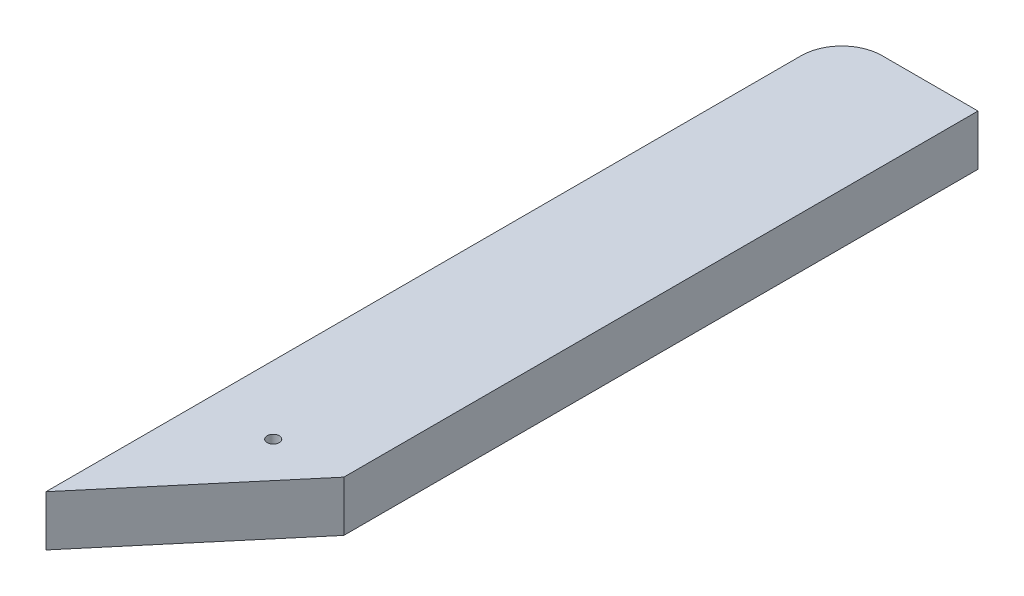
SolidWorks part; units mm, degrees
ref_plane "Front Plane" through (0, 0, 0) normal (0, 0, 1) x (1, 0, 0)
ref_plane "Top Plane" through (0, 0, 0) normal (0, 1, 0) x (1, 0, 0)
ref_plane "Right Plane" through (0, 0, 0) normal (1, 0, 0) x (0, 0, -1)
sketch "Sketch1" plane through (0, 0, 0) normal (0, 1, 0) x (1, 0, 0)
  line L0 (67.5, 0) -> (0, 0)
  line L1 (0, 0) -> (0, -394.0163)
  line L2 (67.5, 0) -> (67.5, -314.0163)
  line L3 (67.5, -314.0163) -> (0, -394.0163)
  line L4 (33.75, -354.0163) -> (33.75, 0) construction
  line L5 (0, -355.2489) -> (67.5, -275.2489) construction
  circle A0 centre (33.75, -315.2489) radius 3
  dimension "D5" = 6
  dimension "D1" = 394.0163
  dimension "D2" = 314.0163
  dimension "D3" = 67.5
  dimension "D4" = 25
extrude "Boss-Extrude1" add sketch "Sketch1" along normal blind 25
fillet "Fillet1" radius 20 1 edges at (0, 12.5, 0)
